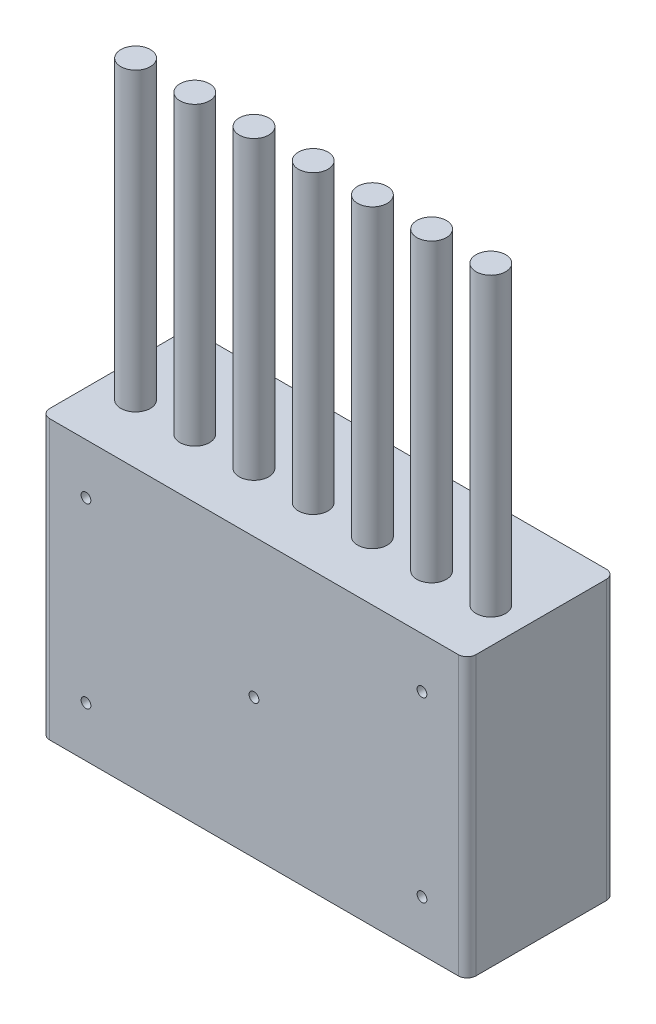
SolidWorks part; units mm, degrees
material "标准件"
ref_plane "前视基准面" through (0, 0, 0) normal (0, 0, 1) x (1, 0, 0)
ref_plane "上视基准面" through (0, 0, 0) normal (0, 1, 0) x (1, 0, 0)
ref_plane "右视基准面" through (0, 0, 0) normal (1, 0, 0) x (0, 0, -1)
sketch "草图1" plane through (0, 0, 0) normal (0, 0, 1) x (1, 0, 0)
  line L1 (-72, -47) -> (72, -47)
  line L2 (-72, -47) -> (-72, 47)
  line L3 (-72, 47) -> (72, 47)
  line L4 (72, -47) -> (72, 47)
  line L5 (-72, -47) -> (72, 47) construction
  line L6 (-72, 47) -> (72, -47) construction
  point P0 (0, 0)
  dimension "D1" = 144
  dimension "D2" = 94
extrude "凸台-拉伸1" add sketch "草图1" along normal blind 50
sketch "草图2" plane through (0, 47, 0) normal (0, 1, 0) x (1, 0, 0)
  line L0 (72, -50) -> (-72, -50) construction
  line L3 (0, -30) -> (20, -30) construction
  line L4 (0, -30) -> (0, -75.3324) construction
  circle A0 centre (0, -30) radius 5
  circle A1 centre (20, -30) radius 5
  circle A2 centre (40, -30) radius 5
  circle A3 centre (60, -30) radius 5
  circle A4 centre (-60, -30) radius 5
  circle A5 centre (-40, -30) radius 5
  circle A6 centre (-20, -30) radius 5
  dimension "D1" = 10
  dimension "D3" = 20
  dimension "D4" = 20
  dimension "D2" = 4
extrude "凸台-拉伸2" add sketch "草图2" along normal blind 100 separate body
fillet "圆角1" radius 3 4 edges at (72, 0, 0) (72, 0, 50) (-72, 0, 0) (-72, 0, 50)
hole_wizard "M4 螺纹孔1" positions "草图3" profile "草图4" tap size "M4" standard "ISO" end condition through all
sketch "草图3" plane through (0, 0, 50) normal (0, 0, 1) x (1, 0, 0)
  line L1 (56.75, -30) -> (-56.75, -30)
  line L2 (56.75, -30) -> (56.75, 30)
  line L3 (56.75, 30) -> (-56.75, 30)
  line L4 (-56.75, -30) -> (-56.75, 30)
  line L5 (56.75, -30) -> (-56.75, 30) construction
  line L6 (56.75, 30) -> (-56.75, -30) construction
  point P0 (-56.75, 30)
  point P3 (0, 0)
  point P8 (56.75, 30)
  point P9 (-56.75, -30)
  point P42 (56.75, -30)
  point P47 (56.75, -30)
  dimension "D1" = 113.5
  dimension "D2" = 60
sketch "草图4" plane through (-56.75, 30, 50) normal (1, 0, 0) x (0, -1, 0)
  line L0 (0, 0) -> (0, 50)
  line L1 (0, 50) -> (1.65, 50)
  line L2 (1.65, 50) -> (1.65, 0)
  line L5 (1.65, 0) -> (0, 0)
  line L11 (0, -6.35) -> (0, 107.95) construction
  dimension "通孔螺纹孔钻头直径" = 3.3
  dimension "通孔螺纹孔钻头深度" = 50
cosmetic thread "孔螺蚊线1" parameters "D2"=4
cosmetic thread "孔螺蚊线2" parameters "D2"=4
cosmetic thread "孔螺蚊线3" parameters "D2"=4
cosmetic thread "孔螺蚊线4" parameters "D2"=4
cosmetic thread "孔螺蚊线5" parameters "D2"=4
